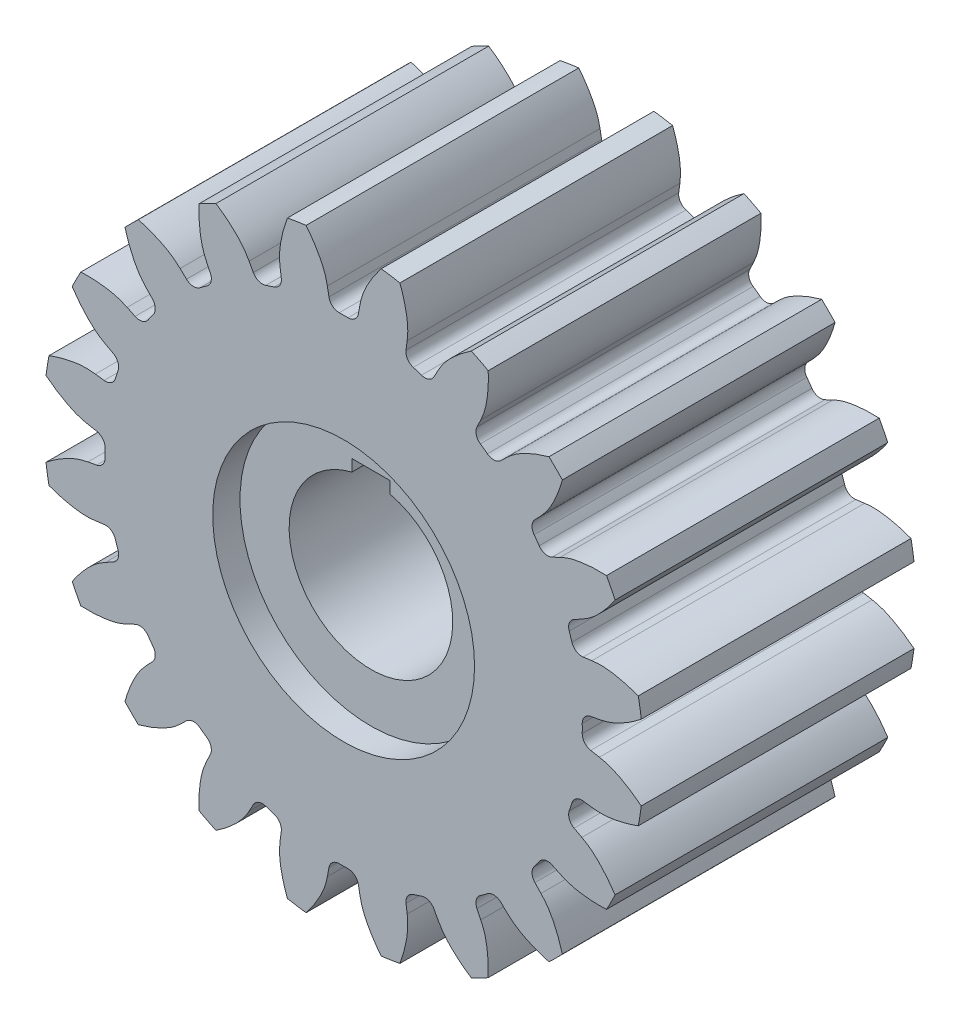
SolidWorks part; units mm, degrees
ref_plane "Front Plane" through (0, 0, 0) normal (0, 0, 1) x (1, 0, 0)
ref_plane "Top Plane" through (0, 0, 0) normal (0, 1, 0) x (1, 0, 0)
ref_plane "Right Plane" through (0, 0, 0) normal (1, 0, 0) x (0, 0, -1)
sketch "Sketch1" plane through (0, 0, 0) normal (0, 0, 1) x (1, 0, 0)
  line L0 (17.5671, 4.5732) -> (18.2072, 4.6592)
  line L1 (18.1205, 1.0792) -> (18.7558, 1.1951)
  line L2 (15.2941, 9.7779) -> (15.8763, 10.0575)
  line L3 (16.9001, 6.6259) -> (17.4685, 6.9325)
  line L4 (11.524, 14.0255) -> (11.9913, 14.4713)
  line L5 (14.0255, 11.524) -> (14.4713, 11.9913)
  line L6 (6.6259, 16.9001) -> (6.9325, 17.4685)
  line L7 (9.7779, 15.2941) -> (10.0575, 15.8763)
  line L8 (1.0792, 18.1205) -> (1.1951, 18.7558)
  line L9 (4.5732, 17.5671) -> (4.6592, 18.2072)
  line L10 (-4.5732, 17.5671) -> (-4.6592, 18.2072)
  line L11 (-1.0792, 18.1205) -> (-1.1951, 18.7558)
  line L12 (-9.7779, 15.2941) -> (-10.0575, 15.8763)
  line L13 (-6.6259, 16.9001) -> (-6.9325, 17.4685)
  line L14 (-14.0255, 11.524) -> (-14.4713, 11.9913)
  line L15 (-11.524, 14.0255) -> (-11.9913, 14.4713)
  line L16 (-16.9001, 6.6259) -> (-17.4685, 6.9325)
  line L17 (-15.2941, 9.7779) -> (-15.8763, 10.0575)
  line L18 (-18.1205, 1.0792) -> (-18.7558, 1.1951)
  line L19 (-17.5671, 4.5732) -> (-18.2072, 4.6592)
  line L20 (-17.5671, -4.5732) -> (-18.2072, -4.6592)
  line L21 (-18.1205, -1.0792) -> (-18.7558, -1.1951)
  line L22 (-15.2941, -9.7779) -> (-15.8763, -10.0575)
  line L23 (-16.9001, -6.6259) -> (-17.4685, -6.9325)
  line L24 (-11.524, -14.0255) -> (-11.9913, -14.4713)
  line L25 (-14.0255, -11.524) -> (-14.4713, -11.9913)
  line L26 (-6.6259, -16.9001) -> (-6.9325, -17.4685)
  line L27 (-9.7779, -15.2941) -> (-10.0575, -15.8763)
  line L28 (-1.0792, -18.1205) -> (-1.1951, -18.7558)
  line L29 (-4.5732, -17.5671) -> (-4.6592, -18.2072)
  line L30 (4.5732, -17.5671) -> (4.6592, -18.2072)
  line L31 (1.0792, -18.1205) -> (1.1951, -18.7558)
  line L32 (9.7779, -15.2941) -> (10.0575, -15.8763)
  line L33 (6.6259, -16.9001) -> (6.9325, -17.4685)
  line L34 (14.0255, -11.524) -> (14.4713, -11.9913)
  line L35 (11.524, -14.0255) -> (11.9913, -14.4713)
  line L36 (16.9001, -6.6259) -> (17.4685, -6.9325)
  line L37 (15.2941, -9.7779) -> (15.8763, -10.0575)
  line L38 (18.1205, -1.0792) -> (18.7558, -1.1951)
  line L39 (17.5671, -4.5732) -> (18.2072, -4.6592)
  arc A0 (16.7389, 5.1047) -> (16.6435, 5.4078) centre (0, 0) ccw
  arc A1 (17.5, 0) -> (17.4971, 0.3177) centre (0, 0) ccw
  arc A2 (21.7291, 3.4416) -> (21.6096, 4.1261) centre (0, 0) ccw
  arc A3 (21.827, 2.7536) -> (21.7291, 3.4416) centre (0, 0) ccw
  arc A4 (16.7389, 5.1047) -> (17.5671, 4.5732) centre (17.4659, 5.3264) ccw
  arc A5 (18.1205, 1.0792) -> (17.4971, 0.3177) centre (18.257, 0.3315) ccw
  arc A6 (14.3422, 10.0275) -> (14.1578, 10.2862) centre (0, 0) ccw
  arc A7 (16.6435, 5.4078) -> (16.5426, 5.7091) centre (0, 0) ccw
  arc A8 (19.6021, 9.9878) -> (19.2769, 10.6018) centre (0, 0) ccw
  arc A9 (19.9078, 9.3638) -> (19.6021, 9.9878) centre (0, 0) ccw
  arc A10 (14.3422, 10.0275) -> (15.2941, 9.7779) centre (14.9651, 10.463) ccw
  arc A11 (16.9001, 6.6259) -> (16.5426, 5.7091) centre (17.261, 5.957) ccw
  arc A12 (10.5416, 13.9687) -> (10.2862, 14.1578) centre (0, 0) ccw
  arc A13 (14.1578, 10.2862) -> (13.9687, 10.5416) centre (0, 0) ccw
  arc A14 (15.5563, 15.5563) -> (15.0573, 16.0399) centre (0, 0) ccw
  arc A15 (16.0399, 15.0573) -> (15.5563, 15.5563) centre (0, 0) ccw
  arc A16 (10.5416, 13.9687) -> (11.524, 14.0255) centre (10.9994, 14.5753) ccw
  arc A17 (14.0255, 11.524) -> (13.9687, 10.5416) centre (14.5753, 10.9994) ccw
  arc A18 (5.7091, 16.5426) -> (5.4078, 16.6435) centre (0, 0) ccw
  arc A19 (10.2862, 14.1578) -> (10.0275, 14.3422) centre (0, 0) ccw
  arc A20 (9.9878, 19.6021) -> (9.3638, 19.9078) centre (0, 0) ccw
  arc A21 (10.6018, 19.2769) -> (9.9878, 19.6021) centre (0, 0) ccw
  arc A22 (5.7091, 16.5426) -> (6.6259, 16.9001) centre (5.957, 17.261) ccw
  arc A23 (9.7779, 15.2941) -> (10.0275, 14.3422) centre (10.463, 14.9651) ccw
  arc A24 (0.3177, 17.4971) -> (0, 17.5) centre (0, 0) ccw
  arc A25 (5.4078, 16.6435) -> (5.1047, 16.7389) centre (0, 0) ccw
  arc A26 (3.4416, 21.7291) -> (2.7536, 21.827) centre (0, 0) ccw
  arc A27 (4.1261, 21.6096) -> (3.4416, 21.7291) centre (0, 0) ccw
  arc A28 (0.3177, 17.4971) -> (1.0792, 18.1205) centre (0.3315, 18.257) ccw
  arc A29 (4.5732, 17.5671) -> (5.1047, 16.7389) centre (5.3264, 17.4659) ccw
  arc A30 (-5.1047, 16.7389) -> (-5.4078, 16.6435) centre (0, 0) ccw
  arc A31 (0, 17.5) -> (-0.3177, 17.4971) centre (0, 0) ccw
  arc A32 (-3.4416, 21.7291) -> (-4.1261, 21.6096) centre (0, 0) ccw
  arc A33 (-2.7536, 21.827) -> (-3.4416, 21.7291) centre (0, 0) ccw
  arc A34 (-5.1047, 16.7389) -> (-4.5732, 17.5671) centre (-5.3264, 17.4659) ccw
  arc A35 (-1.0792, 18.1205) -> (-0.3177, 17.4971) centre (-0.3315, 18.257) ccw
  arc A36 (-10.0275, 14.3422) -> (-10.2862, 14.1578) centre (0, 0) ccw
  arc A37 (-5.4078, 16.6435) -> (-5.7091, 16.5426) centre (0, 0) ccw
  arc A38 (-9.9878, 19.6021) -> (-10.6018, 19.2769) centre (0, 0) ccw
  arc A39 (-9.3638, 19.9078) -> (-9.9878, 19.6021) centre (0, 0) ccw
  arc A40 (-10.0275, 14.3422) -> (-9.7779, 15.2941) centre (-10.463, 14.9651) ccw
  arc A41 (-6.6259, 16.9001) -> (-5.7091, 16.5426) centre (-5.957, 17.261) ccw
  arc A42 (-13.9687, 10.5416) -> (-14.1578, 10.2862) centre (0, 0) ccw
  arc A43 (-10.2862, 14.1578) -> (-10.5416, 13.9687) centre (0, 0) ccw
  arc A44 (-15.5563, 15.5563) -> (-16.0399, 15.0573) centre (0, 0) ccw
  arc A45 (-15.0573, 16.0399) -> (-15.5563, 15.5563) centre (0, 0) ccw
  arc A46 (-13.9687, 10.5416) -> (-14.0255, 11.524) centre (-14.5753, 10.9994) ccw
  arc A47 (-11.524, 14.0255) -> (-10.5416, 13.9687) centre (-10.9994, 14.5753) ccw
  arc A48 (-16.5426, 5.7091) -> (-16.6435, 5.4078) centre (0, 0) ccw
  arc A49 (-14.1578, 10.2862) -> (-14.3422, 10.0275) centre (0, 0) ccw
  arc A50 (-19.6021, 9.9878) -> (-19.9078, 9.3638) centre (0, 0) ccw
  arc A51 (-19.2769, 10.6018) -> (-19.6021, 9.9878) centre (0, 0) ccw
  arc A52 (-16.5426, 5.7091) -> (-16.9001, 6.6259) centre (-17.261, 5.957) ccw
  arc A53 (-15.2941, 9.7779) -> (-14.3422, 10.0275) centre (-14.9651, 10.463) ccw
  arc A54 (-17.4971, 0.3177) -> (-17.5, 0) centre (0, 0) ccw
  arc A55 (-16.6435, 5.4078) -> (-16.7389, 5.1047) centre (0, 0) ccw
  arc A56 (-21.7291, 3.4416) -> (-21.827, 2.7536) centre (0, 0) ccw
  arc A57 (-21.6096, 4.1261) -> (-21.7291, 3.4416) centre (0, 0) ccw
  arc A58 (-17.4971, 0.3177) -> (-18.1205, 1.0792) centre (-18.257, 0.3315) ccw
  arc A59 (-17.5671, 4.5732) -> (-16.7389, 5.1047) centre (-17.4659, 5.3264) ccw
  arc A60 (-16.7389, -5.1047) -> (-16.6435, -5.4078) centre (0, 0) ccw
  arc A61 (-17.5, 0) -> (-17.4971, -0.3177) centre (0, 0) ccw
  arc A62 (-21.7291, -3.4416) -> (-21.6096, -4.1261) centre (0, 0) ccw
  arc A63 (-21.827, -2.7536) -> (-21.7291, -3.4416) centre (0, 0) ccw
  arc A64 (-16.7389, -5.1047) -> (-17.5671, -4.5732) centre (-17.4659, -5.3264) ccw
  arc A65 (-18.1205, -1.0792) -> (-17.4971, -0.3177) centre (-18.257, -0.3315) ccw
  arc A66 (-14.3422, -10.0275) -> (-14.1578, -10.2862) centre (0, 0) ccw
  arc A67 (-16.6435, -5.4078) -> (-16.5426, -5.7091) centre (0, 0) ccw
  arc A68 (-19.6021, -9.9878) -> (-19.2769, -10.6018) centre (0, 0) ccw
  arc A69 (-19.9078, -9.3638) -> (-19.6021, -9.9878) centre (0, 0) ccw
  arc A70 (-14.3422, -10.0275) -> (-15.2941, -9.7779) centre (-14.9651, -10.463) ccw
  arc A71 (-16.9001, -6.6259) -> (-16.5426, -5.7091) centre (-17.261, -5.957) ccw
  arc A72 (-10.5416, -13.9687) -> (-10.2862, -14.1578) centre (0, 0) ccw
  arc A73 (-14.1578, -10.2862) -> (-13.9687, -10.5416) centre (0, 0) ccw
  arc A74 (-15.5563, -15.5563) -> (-15.0573, -16.0399) centre (0, 0) ccw
  arc A75 (-16.0399, -15.0573) -> (-15.5563, -15.5563) centre (0, 0) ccw
  arc A76 (-10.5416, -13.9687) -> (-11.524, -14.0255) centre (-10.9994, -14.5753) ccw
  arc A77 (-14.0255, -11.524) -> (-13.9687, -10.5416) centre (-14.5753, -10.9994) ccw
  arc A78 (-5.7091, -16.5426) -> (-5.4078, -16.6435) centre (0, 0) ccw
  arc A79 (-10.2862, -14.1578) -> (-10.0275, -14.3422) centre (0, 0) ccw
  arc A80 (-9.9878, -19.6021) -> (-9.3638, -19.9078) centre (0, 0) ccw
  arc A81 (-10.6018, -19.2769) -> (-9.9878, -19.6021) centre (0, 0) ccw
  arc A82 (-5.7091, -16.5426) -> (-6.6259, -16.9001) centre (-5.957, -17.261) ccw
  arc A83 (-9.7779, -15.2941) -> (-10.0275, -14.3422) centre (-10.463, -14.9651) ccw
  arc A84 (-0.3177, -17.4971) -> (0, -17.5) centre (0, 0) ccw
  arc A85 (-5.4078, -16.6435) -> (-5.1047, -16.7389) centre (0, 0) ccw
  arc A86 (-3.4416, -21.7291) -> (-2.7536, -21.827) centre (0, 0) ccw
  arc A87 (-4.1261, -21.6096) -> (-3.4416, -21.7291) centre (0, 0) ccw
  arc A88 (-0.3177, -17.4971) -> (-1.0792, -18.1205) centre (-0.3315, -18.257) ccw
  arc A89 (-4.5732, -17.5671) -> (-5.1047, -16.7389) centre (-5.3264, -17.4659) ccw
  arc A90 (5.1047, -16.7389) -> (5.4078, -16.6435) centre (0, 0) ccw
  arc A91 (0, -17.5) -> (0.3177, -17.4971) centre (0, 0) ccw
  arc A92 (3.4416, -21.7291) -> (4.1261, -21.6096) centre (0, 0) ccw
  arc A93 (2.7536, -21.827) -> (3.4416, -21.7291) centre (0, 0) ccw
  arc A94 (5.1047, -16.7389) -> (4.5732, -17.5671) centre (5.3264, -17.4659) ccw
  arc A95 (1.0792, -18.1205) -> (0.3177, -17.4971) centre (0.3315, -18.257) ccw
  arc A96 (10.0275, -14.3422) -> (10.2862, -14.1578) centre (0, 0) ccw
  arc A97 (5.4078, -16.6435) -> (5.7091, -16.5426) centre (0, 0) ccw
  arc A98 (9.9878, -19.6021) -> (10.6018, -19.2769) centre (0, 0) ccw
  arc A99 (9.3638, -19.9078) -> (9.9878, -19.6021) centre (0, 0) ccw
  arc A100 (10.0275, -14.3422) -> (9.7779, -15.2941) centre (10.463, -14.9651) ccw
  arc A101 (6.6259, -16.9001) -> (5.7091, -16.5426) centre (5.957, -17.261) ccw
  arc A102 (13.9687, -10.5416) -> (14.1578, -10.2862) centre (0, 0) ccw
  arc A103 (10.2862, -14.1578) -> (10.5416, -13.9687) centre (0, 0) ccw
  arc A104 (15.5563, -15.5563) -> (16.0399, -15.0573) centre (0, 0) ccw
  arc A105 (15.0573, -16.0399) -> (15.5563, -15.5563) centre (0, 0) ccw
  arc A106 (13.9687, -10.5416) -> (14.0255, -11.524) centre (14.5753, -10.9994) ccw
  arc A107 (11.524, -14.0255) -> (10.5416, -13.9687) centre (10.9994, -14.5753) ccw
  arc A108 (16.5426, -5.7091) -> (16.6435, -5.4078) centre (0, 0) ccw
  arc A109 (14.1578, -10.2862) -> (14.3422, -10.0275) centre (0, 0) ccw
  arc A110 (19.6021, -9.9878) -> (19.9078, -9.3638) centre (0, 0) ccw
  arc A111 (19.2769, -10.6018) -> (19.6021, -9.9878) centre (0, 0) ccw
  arc A112 (16.5426, -5.7091) -> (16.9001, -6.6259) centre (17.261, -5.957) ccw
  arc A113 (15.2941, -9.7779) -> (14.3422, -10.0275) centre (14.9651, -10.463) ccw
  arc A114 (17.4971, -0.3177) -> (17.5, 0) centre (0, 0) ccw
  arc A115 (16.6435, -5.4078) -> (16.7389, -5.1047) centre (0, 0) ccw
  arc A116 (21.7291, -3.4416) -> (21.827, -2.7536) centre (0, 0) ccw
  arc A117 (21.6096, -4.1261) -> (21.7291, -3.4416) centre (0, 0) ccw
  arc A118 (17.4971, -0.3177) -> (18.1205, -1.0792) centre (18.257, -0.3315) ccw
  arc A119 (17.5671, -4.5732) -> (16.7389, -5.1047) centre (17.4659, -5.3264) ccw
  spline S0 degree 3 poles (18.2072, 4.6592) (18.477, 4.6955) (19.0358, 4.7288) (19.8837, 4.6199) (20.7487, 4.4222) (21.3226, 4.235) (21.6096, 4.1261) knots 0 0 0 0 44.621092 91.187357 139.632096 189.949047 189.949047 189.949047 189.949047 weights 1 1 1 1 1 1 1
  spline S1 degree 3 poles (18.7558, 1.1951) (19.0236, 1.244) (19.5653, 1.385) (20.3382, 1.7506) (21.0998, 2.206) (21.5877, 2.5613) (21.827, 2.7536) knots 0 0 0 0 48.786984 99.700744 152.668356 207.682972 207.682972 207.682972 207.682972 weights 1 1 1 1 1 1 1
  spline S2 degree 3 poles (15.8763, 10.0575) (16.1216, 10.1753) (16.6428, 10.3797) (17.4829, 10.5382) (18.3667, 10.6174) (18.9703, 10.6168) (19.2769, 10.6018) knots 0 0 0 0 37.395678 76.421551 117.02172 159.190936 159.190936 159.190936 159.190936 weights 1 1 1 1 1 1 1
  spline S3 degree 3 poles (17.4685, 6.9325) (17.7081, 7.0618) (18.1798, 7.3633) (18.8018, 7.9498) (19.3854, 8.6182) (19.7396, 9.107) (19.9078, 9.3638) knots 0 0 0 0 40.49406 82.753383 126.717438 172.380543 172.380543 172.380543 172.380543 weights 1 1 1 1 1 1 1
  spline S4 degree 3 poles (11.9913, 14.4713) (12.1882, 14.6592) (12.6207, 15.0146) (13.3708, 15.4249) (14.1868, 15.7734) (14.7611, 15.9593) (15.0573, 16.0399) knots 0 0 0 0 35.757785 73.074364 111.896287 152.218534 152.218534 152.218534 152.218534 weights 1 1 1 1 1 1 1
  spline S5 degree 3 poles (14.4713, 11.9913) (14.6592, 12.1882) (15.0146, 12.6207) (15.4249, 13.3708) (15.7734, 14.1868) (15.9593, 14.7611) (16.0399, 15.0573) knots 0 0 0 0 35.955531 73.478477 112.51509 153.060326 153.060326 153.060326 153.060326 weights 1 1 1 1 1 1 1
  spline S6 degree 3 poles (6.9325, 17.4685) (7.0618, 17.7081) (7.3633, 18.1798) (7.9498, 18.8018) (8.6182, 19.3854) (9.107, 19.7396) (9.3638, 19.9078) knots 0 0 0 0 41.056954 83.903709 128.478893 174.776745 174.776745 174.776745 174.776745 weights 1 1 1 1 1 1 1
  spline S7 degree 3 poles (10.0575, 15.8763) (10.1753, 16.1216) (10.3797, 16.6428) (10.5382, 17.4829) (10.6174, 18.3667) (10.6168, 18.9703) (10.6018, 19.2769) knots 0 0 0 0 38.160336 77.984201 119.414552 162.446035 162.446035 162.446035 162.446035 weights 1 1 1 1 1 1 1
  spline S8 degree 3 poles (1.1951, 18.7558) (1.244, 19.0236) (1.385, 19.5653) (1.7506, 20.3382) (2.206, 21.0998) (2.5613, 21.5877) (2.7536, 21.827) knots 0 0 0 0 50.061411 102.305155 156.656402 213.108124 213.108124 213.108124 213.108124 weights 1 1 1 1 1 1 1
  spline S9 degree 3 poles (4.6592, 18.2072) (4.6955, 18.477) (4.7288, 19.0358) (4.6199, 19.8837) (4.4222, 20.7487) (4.235, 21.3226) (4.1261, 21.6096) knots 0 0 0 0 46.029666 94.065908 144.039924 195.945251 195.945251 195.945251 195.945251 weights 1 1 1 1 1 1 1
  spline S10 degree 3 poles (-4.6592, 18.2072) (-4.6955, 18.477) (-4.7288, 19.0358) (-4.6199, 19.8837) (-4.4222, 20.7487) (-4.235, 21.3226) (-4.1261, 21.6096) knots 0 0 0 0 58.365767 119.275879 182.643095 248.45922 248.45922 248.45922 248.45922 weights 1 1 1 1 1 1 1
  spline S11 degree 3 poles (-1.1951, 18.7558) (-1.244, 19.0236) (-1.385, 19.5653) (-1.7506, 20.3382) (-2.206, 21.0998) (-2.5613, 21.5877) (-2.7536, 21.827) knots 0 0 0 0 55.007404 112.412751 172.13382 234.162889 234.162889 234.162889 234.162889 weights 1 1 1 1 1 1 1
  spline S12 degree 3 poles (-10.0575, 15.8763) (-10.1753, 16.1216) (-10.3797, 16.6428) (-10.5382, 17.4829) (-10.6174, 18.3667) (-10.6168, 18.9703) (-10.6018, 19.2769) knots 0 0 0 0 63.7318 130.241867 199.434938 271.302067 271.302067 271.302067 271.302067 weights 1 1 1 1 1 1 1
  spline S13 degree 3 poles (-6.9325, 17.4685) (-7.0618, 17.7081) (-7.3633, 18.1798) (-7.9498, 18.8018) (-8.6182, 19.3854) (-9.107, 19.7396) (-9.3638, 19.9078) knots 0 0 0 0 61.882296 126.462234 193.647314 263.428851 263.428851 263.428851 263.428851 weights 1 1 1 1 1 1 1
  spline S14 degree 3 poles (-14.4713, 11.9913) (-14.6592, 12.1882) (-15.0146, 12.6207) (-15.4249, 13.3708) (-15.7734, 14.1868) (-15.9593, 14.7611) (-16.0399, 15.0573) knots 0 0 0 0 65.184441 133.210475 203.980667 277.485867 277.485867 277.485867 277.485867 weights 1 1 1 1 1 1 1
  spline S15 degree 3 poles (-11.9913, 14.4713) (-12.1882, 14.6592) (-12.6207, 15.0146) (-13.3708, 15.4249) (-14.1868, 15.7734) (-14.7611, 15.9593) (-15.0573, 16.0399) knots 0 0 0 0 65.189629 133.221078 203.996902 277.507952 277.507952 277.507952 277.507952 weights 1 1 1 1 1 1 1
  spline S16 degree 3 poles (-17.4685, 6.9325) (-17.7081, 7.0618) (-18.1798, 7.3633) (-18.8018, 7.9498) (-19.3854, 8.6182) (-19.7396, 9.107) (-19.9078, 9.3638) knots 0 0 0 0 62.5388 127.803862 195.701703 266.223547 266.223547 266.223547 266.223547 weights 1 1 1 1 1 1 1
  spline S17 degree 3 poles (-15.8763, 10.0575) (-16.1216, 10.1753) (-16.6428, 10.3797) (-17.4829, 10.5382) (-18.3667, 10.6174) (-18.9703, 10.6168) (-19.2769, 10.6018) knots 0 0 0 0 64.400605 131.608632 201.52782 274.149126 274.149126 274.149126 274.149126 weights 1 1 1 1 1 1 1
  spline S18 degree 3 poles (-18.7558, 1.1951) (-19.0236, 1.244) (-19.5653, 1.385) (-20.3382, 1.7506) (-21.0998, 2.206) (-21.5877, 2.5613) (-21.827, 2.7536) knots 0 0 0 0 56.345383 115.147037 176.320739 239.858579 239.858579 239.858579 239.858579 weights 1 1 1 1 1 1 1
  spline S19 degree 3 poles (-18.2072, 4.6592) (-18.477, 4.6955) (-19.0358, 4.7288) (-19.8837, 4.6199) (-20.7487, 4.4222) (-21.3226, 4.235) (-21.6096, 4.1261) knots 0 0 0 0 59.72248 122.048448 186.888635 254.234657 254.234657 254.234657 254.234657 weights 1 1 1 1 1 1 1
  spline S20 degree 3 poles (-18.2072, -4.6592) (-18.477, -4.6955) (-19.0358, -4.7288) (-19.8837, -4.6199) (-20.7487, -4.4222) (-21.3226, -4.235) (-21.6096, -4.1261) knots 0 0 0 0 48.099347 98.295494 150.516544 204.755746 204.755746 204.755746 204.755746 weights 1 1 1 1 1 1 1
  spline S21 degree 3 poles (-18.7558, -1.1951) (-19.0236, -1.244) (-19.5653, -1.385) (-20.3382, -1.7506) (-21.0998, -2.206) (-21.5877, -2.5613) (-21.827, -2.7536) knots 0 0 0 0 52.173739 106.621893 163.266477 222.100165 222.100165 222.100165 222.100165 weights 1 1 1 1 1 1 1
  spline S22 degree 3 poles (-15.8763, -10.0575) (-16.1216, -10.1753) (-16.6428, -10.3797) (-17.4829, -10.5382) (-18.3667, -10.6174) (-18.9703, -10.6168) (-19.2769, -10.6018) knots 0 0 0 0 40.908743 83.600826 128.015099 174.145821 174.145821 174.145821 174.145821 weights 1 1 1 1 1 1 1
  spline S23 degree 3 poles (-17.4685, -6.9325) (-17.7081, -7.0618) (-18.1798, -7.3633) (-18.8018, -7.9498) (-19.3854, -8.6182) (-19.7396, -9.107) (-19.9078, -9.3638) knots 0 0 0 0 44.029427 89.978235 137.780609 187.430368 187.430368 187.430368 187.430368 weights 1 1 1 1 1 1 1
  spline S24 degree 3 poles (-11.9913, -14.4713) (-12.1882, -14.6592) (-12.6207, -15.0146) (-13.3708, -15.4249) (-14.1868, -15.7734) (-14.7611, -15.9593) (-15.0573, -16.0399) knots 0 0 0 0 38.792627 79.276345 121.393169 165.137654 165.137654 165.137654 165.137654 weights 1 1 1 1 1 1 1
  spline S25 degree 3 poles (-14.4713, -11.9913) (-14.6592, -12.1882) (-15.0146, -12.6207) (-15.4249, -13.3708) (-15.7734, -14.1868) (-15.9593, -14.7611) (-16.0399, -15.0573) knots 0 0 0 0 39.262663 80.236908 122.864046 167.138566 167.138566 167.138566 167.138566 weights 1 1 1 1 1 1 1
  spline S26 degree 3 poles (-6.9325, -17.4685) (-7.0618, -17.7081) (-7.3633, -18.1798) (-7.9498, -18.8018) (-8.6182, -19.3854) (-9.107, -19.7396) (-9.3638, -19.9078) knots 0 0 0 0 42.798548 87.462819 133.928838 182.190598 182.190598 182.190598 182.190598 weights 1 1 1 1 1 1 1
  spline S27 degree 3 poles (-10.0575, -15.8763) (-10.1753, -16.1216) (-10.3797, -16.6428) (-10.5382, -17.4829) (-10.6174, -18.3667) (-10.6168, -18.9703) (-10.6018, -19.2769) knots 0 0 0 0 40.519447 82.805262 126.79688 172.488612 172.488612 172.488612 172.488612 weights 1 1 1 1 1 1 1
  spline S28 degree 3 poles (-1.1951, -18.7558) (-1.244, -19.0236) (-1.385, -19.5653) (-1.7506, -20.3382) (-2.206, -21.0998) (-2.5613, -21.5877) (-2.7536, -21.827) knots 0 0 0 0 50.397015 102.990994 157.706603 214.53677 214.53677 214.53677 214.53677 weights 1 1 1 1 1 1 1
  spline S29 degree 3 poles (-4.6592, -18.2072) (-4.6955, -18.477) (-4.7288, -19.0358) (-4.6199, -19.8837) (-4.4222, -20.7487) (-4.235, -21.3226) (-4.1261, -21.6096) knots 0 0 0 0 46.923242 95.892014 146.836177 199.749145 199.749145 199.749145 199.749145 weights 1 1 1 1 1 1 1
  spline S30 degree 3 poles (4.6592, -18.2072) (4.6955, -18.477) (4.7288, -19.0358) (4.6199, -19.8837) (4.4222, -20.7487) (4.235, -21.3226) (4.1261, -21.6096) knots 0 0 0 0 57.630301 117.772886 180.341612 245.328389 245.328389 245.328389 245.328389 weights 1 1 1 1 1 1 1
  spline S31 degree 3 poles (1.1951, -18.7558) (1.244, -19.0236) (1.385, -19.5653) (1.7506, -20.3382) (2.206, -21.0998) (2.5613, -21.5877) (2.7536, -21.827) knots 0 0 0 0 54.699372 111.78326 171.169902 232.851619 232.851619 232.851619 232.851619 weights 1 1 1 1 1 1 1
  spline S32 degree 3 poles (10.0575, -15.8763) (10.1753, -16.1216) (10.3797, -16.6428) (10.5382, -17.4829) (10.6174, -18.3667) (10.6168, -18.9703) (10.6018, -19.2769) knots 0 0 0 0 62.154254 127.018006 194.49835 264.58656 264.58656 264.58656 264.58656 weights 1 1 1 1 1 1 1
  spline S33 degree 3 poles (6.9325, -17.4685) (7.0618, -17.7081) (7.3633, -18.1798) (7.9498, -18.8018) (8.6182, -19.3854) (9.107, -19.7396) (9.3638, -19.9078) knots 0 0 0 0 60.648108 123.940056 189.785189 258.174995 258.174995 258.174995 258.174995 weights 1 1 1 1 1 1 1
  spline S34 degree 3 poles (14.4713, -11.9913) (14.6592, -12.1882) (15.0146, -12.6207) (15.4249, -13.3708) (15.7734, -14.1868) (15.9593, -14.7611) (16.0399, -15.0573) knots 0 0 0 0 62.925888 128.594911 196.913011 267.871353 267.871353 267.871353 267.871353 weights 1 1 1 1 1 1 1
  spline S35 degree 3 poles (11.9913, -14.4713) (12.1882, -14.6592) (12.6207, -15.0146) (13.3708, -15.4249) (14.1868, -15.7734) (14.7611, -15.9593) (15.0573, -16.0399) knots 0 0 0 0 63.209035 129.173549 197.79906 269.076694 269.076694 269.076694 269.076694 weights 1 1 1 1 1 1 1
  spline S36 degree 3 poles (17.4685, -6.9325) (17.7081, -7.0618) (18.1798, -7.3633) (18.8018, -7.9498) (19.3854, -8.6182) (19.7396, -9.107) (19.9078, -9.3638) knots 0 0 0 0 59.737721 122.079595 186.936329 254.299538 254.299538 254.299538 254.299538 weights 1 1 1 1 1 1 1
  spline S37 degree 3 poles (15.8763, -10.0575) (16.1216, -10.1753) (16.6428, -10.3797) (17.4829, -10.5382) (18.3667, -10.6174) (18.9703, -10.6168) (19.2769, -10.6018) knots 0 0 0 0 61.817188 126.32918 193.443574 263.151693 263.151693 263.151693 263.151693 weights 1 1 1 1 1 1 1
  spline S38 degree 3 poles (18.7558, -1.1951) (19.0236, -1.244) (19.5653, -1.385) (20.3382, -1.7506) (21.0998, -2.206) (21.5877, -2.5613) (21.827, -2.7536) knots 0 0 0 0 53.13399 108.584256 166.271376 226.187891 226.187891 226.187891 226.187891 weights 1 1 1 1 1 1 1
  spline S39 degree 3 poles (18.2072, -4.6592) (18.477, -4.6955) (19.0358, -4.7288) (19.8837, -4.6199) (20.7487, -4.4222) (21.3226, -4.235) (21.6096, -4.1261) knots 0 0 0 0 56.669331 115.809055 177.334465 241.237605 241.237605 241.237605 241.237605 weights 1 1 1 1 1 1 1
extrude "Boss-Extrude1" add sketch "Sketch1" along normal mid plane 20
sketch "Sketch6" plane through (0, 0, -10) normal (0, 0, -1) x (-1, 0, 0)
  circle A0 centre (0, 0) radius 6
  circle A1 centre (0, 0) radius 9.6
  dimension "D1" = 19.2
  dimension "D2" = 12
extrude "Cut-Extrude2" cut sketch "Sketch6" against normal blind 2
sketch "Sketch7" plane through (0, 0, 10) normal (0, 0, 1) x (1, 0, 0)
  circle A0 centre (0, 0) radius 6
  circle A1 centre (0, 0) radius 9.6
  dimension "D1" = 12
  dimension "D2" = 19.2
extrude "Cut-Extrude3" cut sketch "Sketch7" against normal blind 2
sketch "Sketch8" plane through (0, 0, 10) normal (0, 0, 1) x (1, 0, 0)
  circle A1 centre (0, 0) radius 6
  circle A2 centre (0, 0) radius 6
  dimension "D1" = 0
extrude "Cut-Extrude4" cut sketch "Sketch8" against normal through all
sketch "Sketch9" plane through (0, 0, 0) normal (0, 0, 1) x (1, 0, 0)
  line L0 (1.4, 6.7) -> (1.4, 5)
  line L1 (1.4, 5) -> (-1.4, 5)
  line L2 (-1.4, 5) -> (-1.4, 6.7)
  line L3 (1.4, 6.7) -> (-1.4, 6.7)
  line L4 (0, 8.3259) -> (0, -0.7668) construction
  dimension "D1" = 5
  dimension "D2" = 1.7
  dimension "D3" = 2.8
extrude "Cut-Extrude5" cut sketch "Sketch9" along normal mid plane 20
sketch "Sketch10" plane through (0, 0, 0) normal (0, 0, 1) x (1, 0, 0)
  circle A0 centre (0, 0) radius 20
  dimension "D1" = 40
sketch "Sketch11" plane through (0, 0, 0) normal (0, 0, 1) x (1, 0, 0)
  line L0 (0, 0) -> (21.7291, 3.4416)
  arc A0 (21.827, 2.7536) -> (21.6096, 4.1261) centre (0, 0) ccw construction
